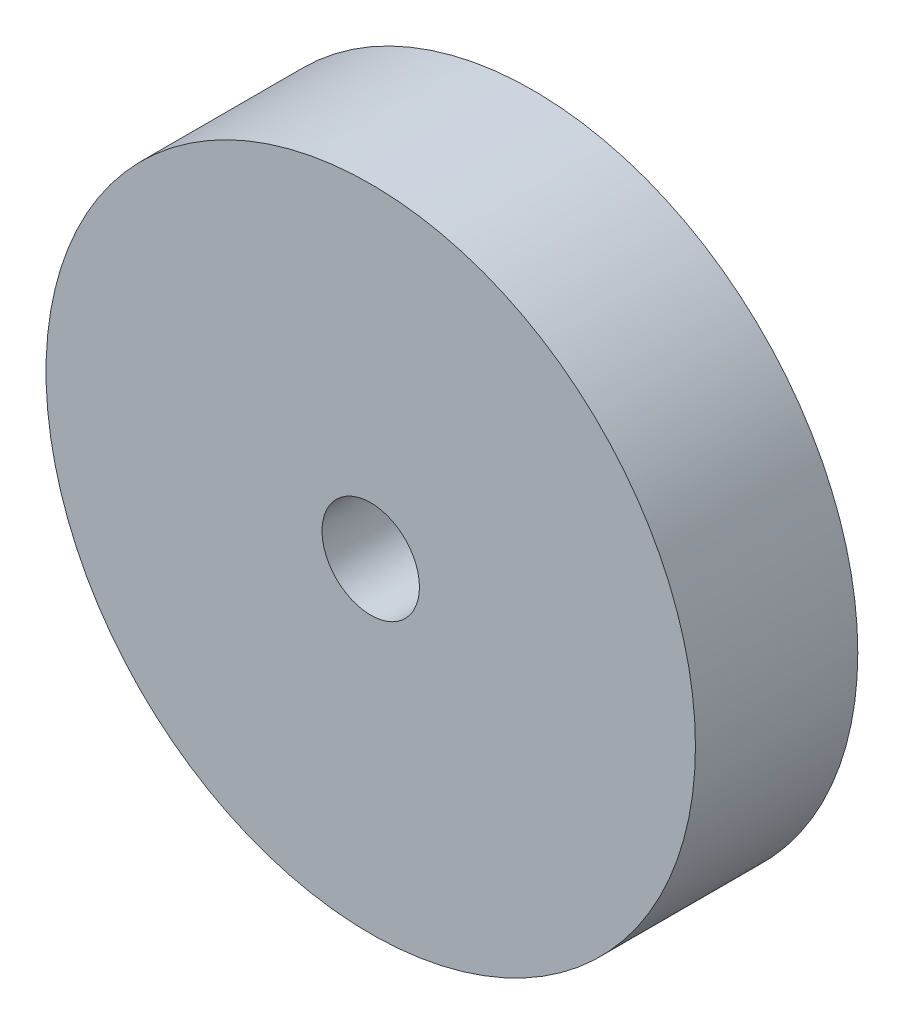
from build123d import *

# Parameters (mm, degrees)
SKETCH_1_W = 17
SKETCH_1_H = 10


with BuildPart() as part:
    # 草图1 → 旋转1 (revolve)
    with BuildSketch(Plane(origin=(0, 0, 0), x_dir=(1, 0, 0), z_dir=(0, 1, 0)), mode=Mode.PRIVATE) as revolve_1_sk:
        with Locations((-11.5, 5)):
            Rectangle(SKETCH_1_W, SKETCH_1_H)
    revolve(revolve_1_sk.sketch.rotate(Axis((0, 0, 129.063142874), (0, 0, -1)), 180), axis=Axis((0, 0, 129.063142874), (0, 0, -1)))


solid = part.part
